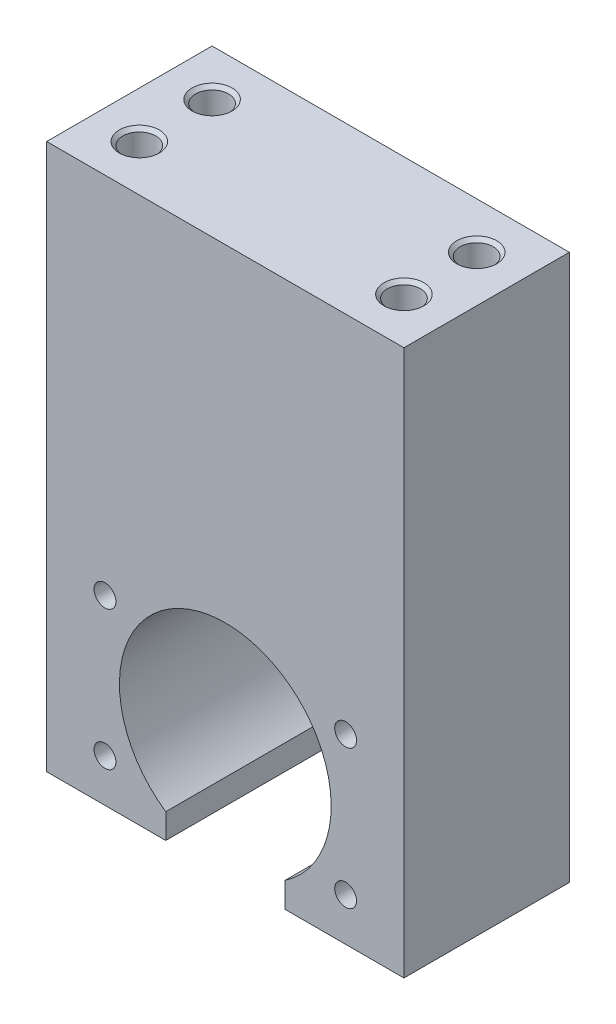
SolidWorks part; units mm, degrees
ref_plane "前视基准面" through (0, 0, 0) normal (0, 0, 1) x (1, 0, 0)
ref_plane "上视基准面" through (0, 0, 0) normal (0, 1, 0) x (1, 0, 0)
ref_plane "右视基准面" through (0, 0, 0) normal (1, 0, 0) x (0, 0, -1)
sketch "草图1" plane through (0, 0, 0) normal (0, 0, 1) x (1, 0, 0)
  line L0 (-27, 65.5) -> (27, 65.5)
  line L1 (27, 65.5) -> (27, -17)
  line L2 (27, -17) -> (9, -17)
  line L3 (9, -17) -> (9, -13.2288)
  line L4 (-27, 65.5) -> (-27, -17)
  line L5 (-27, -17) -> (-9, -17)
  line L6 (-9, -17) -> (-9, -13.2288)
  arc A0 (9, -13.2288) -> (-9, -13.2288) centre (0, 0) ccw
extrude "凸台-拉伸1" add sketch "草图1" along normal mid plane 25
hole_wizard "M4 螺纹孔1" positions "草图3" profile "草图2" tap size "M4" standard "GB"
sketch "草图3" plane through (0, 0, 12.5) normal (0, 0, 1) x (1, 0, 0)
  circle A0 centre (18.1865, 10.5) radius 2.25 construction
  circle A1 centre (18.1865, -10.5) radius 2.25 construction
  circle A2 centre (-18.1865, -10.5) radius 2.25 construction
  circle A3 centre (-18.1865, 10.5) radius 2.25 construction
  point P1 (18.1865, 10.5)
  point P5 (18.1865, -10.5)
  point P9 (-18.1865, -10.5)
  point P13 (-18.1865, 10.5)
cosmetic thread "孔螺蚊线1" parameters "D1"=6, "D2"=4
cosmetic thread "孔螺蚊线2" parameters "D1"=6, "D2"=4
cosmetic thread "孔螺蚊线3" parameters "D1"=6, "D2"=4
cosmetic thread "孔螺蚊线4" parameters "D1"=6, "D2"=4
sketch "草图2" plane through (18.1865, 10.5, 12.5) normal (1, 0, 0) x (0, -1, 0)
  line L0 (0, 0) -> (0, 10.4914)
  line L1 (0, 10.4914) -> (1.65, 9.5)
  line L2 (1.65, 9.5) -> (1.65, 0)
  line L5 (1.65, 0) -> (0, 0)
  line L10 (0, 10.4914) -> (-1.65, 9.5) construction
  line L11 (0, -6.35) -> (0, 107.95) construction
  dimension "螺纹孔钻头直径" = 3.3
  dimension "螺纹孔钻头深度" = 9.5
  dimension "导头角度" = 118
sketch "草图4" plane through (0, 65.5, 0) normal (0, 1, 0) x (1, 0, 0)
  line L0 (27, -12.5) -> (27, 12.5) construction
  line L1 (-20, -5.5) -> (20, -5.5)
  line L2 (-20, -5.5) -> (-20, 5.5)
  line L3 (-20, 5.5) -> (20, 5.5)
  line L4 (20, -5.5) -> (20, 5.5)
  line L5 (-20, -5.5) -> (20, 5.5) construction
  line L6 (-20, 5.5) -> (20, -5.5) construction
  line L7 (27, -12.5) -> (-27, -12.5) construction
  point P0 (0, 0)
  dimension "D1" = 7
  dimension "D2" = 7
hole_wizard "M6 螺纹孔1" positions "3D草图1" profile "草图5" tap size "M6" standard "GB"
sketch3d "3D草图1"
  point P0 (-20, 65.5, 5.5)
  point P3 (-20, 65.5, -5.5)
  point P6 (20, 65.5, -5.5)
  point P9 (20, 65.5, 5.5)
sketch "草图5" plane through (-20, 65.5, 5.5) normal (1, 0, 0) x (0, 0, 1)
  line L0 (0, 0) -> (0, 13.5022)
  line L1 (0, 13.5022) -> (2.5, 12)
  line L2 (2.5, 12) -> (2.5, 0.525)
  line L3 (2.5, 0.525) -> (3.025, 0)
  line L5 (3.025, 0) -> (0, 0)
  line L6 (-2.5, 0.525) -> (-3.025, 0) construction
  line L10 (0, 13.5022) -> (-2.5, 12) construction
  line L11 (0, -6.35) -> (0, 107.95) construction
  dimension "螺纹孔钻头直径" = 5
  dimension "螺纹孔钻头深度" = 12
  dimension "近端锥形沉头孔直径" = 6.05
  dimension "近端锥形沉头孔角度" = 90
  dimension "导头角度" = 118
cosmetic thread "孔螺蚊线5" parameters "D1"=8, "D2"=6
cosmetic thread "孔螺蚊线6" parameters "D1"=8, "D2"=6
cosmetic thread "孔螺蚊线7" parameters "D1"=8, "D2"=6
cosmetic thread "孔螺蚊线8" parameters "D1"=8, "D2"=6
equation "\"D3@草图1\"=\"D2@草图1\""
